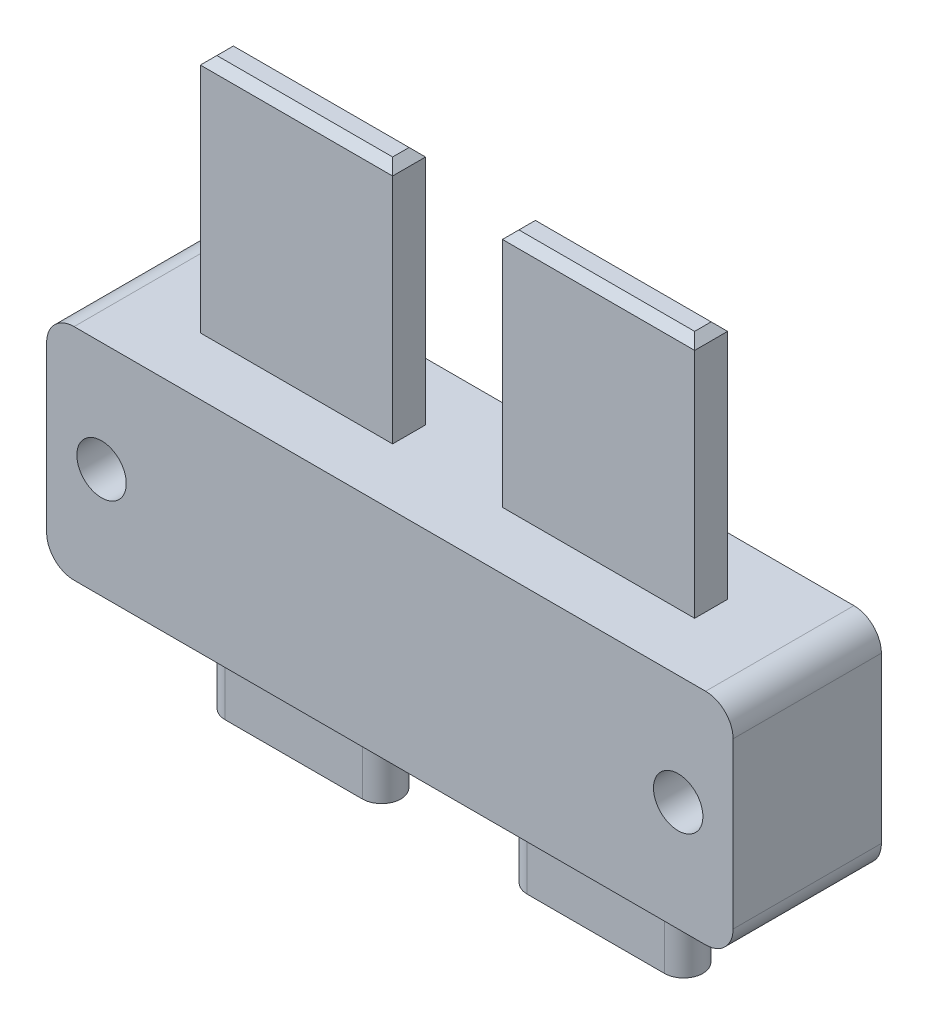
from build123d import *

# Parameters (mm, degrees)
SKETCH_1_W      = 25
SKETCH_1_H      = 8
SKETCH_1_R      = 0.9
EXTRUDE_1_DEPTH = 5.4
EXTRUDE_2_DEPTH = 3.65
SKETCH_3_W      = 7
SKETCH_3_H      = 1.2
EXTRUDE_3_DEPTH = 8.75
CHAMFER_1_SIZE  = 0.3
FILLET_1_R      = 1


with BuildPart() as part:
    # 草图1 → 凸台-拉伸1 (new body)
    with BuildSketch(Plane.XY):
        Rectangle(SKETCH_1_W, SKETCH_1_H)
        with Locations(Location((10.5, 0, 0), (0, 0, 180))):
            Circle(SKETCH_1_R, mode=Mode.SUBTRACT)
        with Locations(Location((-10.5, 0, 0), (0, 0, 180))):
            Circle(SKETCH_1_R, mode=Mode.SUBTRACT)
    extrude(amount=EXTRUDE_1_DEPTH)

    # 草图2 → 凸台-拉伸2 (add)
    with BuildSketch(Plane(origin=(0, -4, 0), x_dir=(-1, 0, 0), z_dir=(0, -1, 0))):
        with BuildLine():
            Line((-3, -3.4), (-8, -3.4))
            ThreePointArc((-8, -3.4), (-8.7, -2.7), (-8, -2))
            Line((-8, -2), (-3, -2))
            ThreePointArc((-3, -2), (-2.3, -2.7), (-3, -3.4))
        make_face()
        with BuildLine():
            Line((3, -3.4), (8, -3.4))
            ThreePointArc((8, -3.4), (8.7, -2.7), (8, -2))
            Line((8, -2), (3, -2))
            ThreePointArc((3, -2), (2.3, -2.7), (3, -3.4))
        make_face()
    extrude(amount=EXTRUDE_2_DEPTH)

    # 草图3 → 凸台-拉伸3 (add)
    with BuildSketch(Plane(origin=(0, 4, 0), x_dir=(1, 0, 0), z_dir=(0, 1, 0))):
        with Locations((5.5, -2.7)):
            Rectangle(SKETCH_3_W, SKETCH_3_H)
        with Locations((-5.5, -2.7)):
            Rectangle(SKETCH_3_W, SKETCH_3_H)
    extrude(amount=EXTRUDE_3_DEPTH)

    # 倒角1
    chamfer_1_edges = [part.edges().sort_by_distance(p)[0] for p in [
        (9, 12.75, 2.7),
        (5.5, 12.75, 2.1),
        (2, 12.75, 2.7),
        (5.5, 12.75, 3.3),
        (-2, 12.75, 2.7),
        (-5.5, 12.75, 2.1),
        (-9, 12.75, 2.7),
        (-5.5, 12.75, 3.3),
    ]]
    chamfer(chamfer_1_edges, length=CHAMFER_1_SIZE)

    # 圆角1
    fillet_1_edges = [part.edges().sort_by_distance(p)[0] for p in [
        (12.5, -4, 2.7),
        (-12.5, -4, 2.7),
        (-12.5, 4, 2.7),
        (12.5, 4, 2.7),
    ]]
    fillet(fillet_1_edges, radius=FILLET_1_R)


solid = part.part
